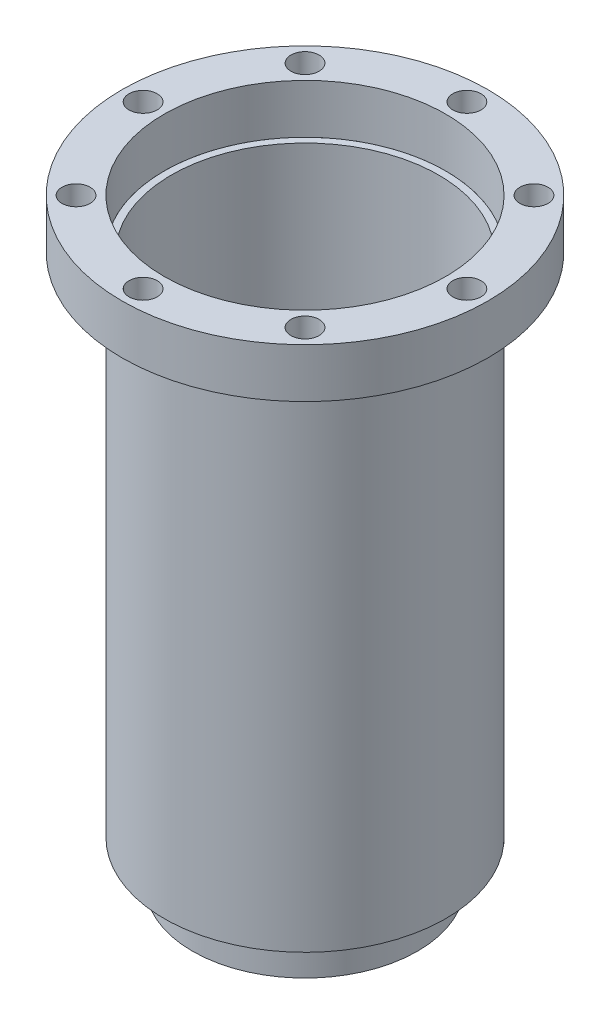
from build123d import *

# Parameters (mm, degrees)
SKETCH1_R               = 100
BOSS_EXTRUDE1_DEPTH     = 360
SHELL1_T                = -10
SKETCH2_R               = 70
CUT_EXTRUDE1_DEPTH      = 300
SKETCH3_R               = 80
SKETCH3_R_2             = 70
BOSS_EXTRUDE2_DEPTH     = 30
SKETCH4_R               = 130
SKETCH4_R_2             = 100
BOSS_EXTRUDE3_DEPTH     = 35
CUT_EXTRUDE3_DEPTH      = 432.161222746
CUT_EXTRUDE3_DEPTH_BACK = 309
SKETCH6_R               = 95
SKETCH6_R_2             = 90
SKETCH7_R               = 10
CUT_EXTRUDE6_DEPTH      = 464.060471213
CIRPATTERN1_COUNT       = 8


with BuildPart() as part:
    # Sketch1 → Boss-Extrude1 (new body)
    with BuildSketch(Plane(origin=(0, 0, 0), x_dir=(1, 0, 0), z_dir=(0, 1, 0))):
        with Locations(Location((0, 0, 0), (0, 0, 90))):
            Circle(SKETCH1_R)
    extrude(amount=BOSS_EXTRUDE1_DEPTH)

    # Shell1
    shell1_openings = [part.faces().sort_by_distance(p)[0] for p in [
        (0, 360, 0),
    ]]
    offset(amount=SHELL1_T, openings=shell1_openings, kind=Kind.INTERSECTION)

    # Sketch2 → Cut-Extrude1 (cut)
    with BuildSketch(Plane(origin=(0, 10, 0), x_dir=(1, 0, 0), z_dir=(0, 1, 0))):
        with Locations(Location((0, 0, 0), (0, 0, 270))):
            Circle(SKETCH2_R)
    extrude(amount=-CUT_EXTRUDE1_DEPTH, mode=Mode.SUBTRACT)

    # Sketch3 → Boss-Extrude2 (add)
    with BuildSketch(Plane.XZ):
        with Locations(Location((0, 0, 0), (0, 0, 90))):
            Circle(SKETCH3_R)
        with Locations(Location((0, 0, 0), (0, 0, 90))):
            Circle(SKETCH3_R_2, mode=Mode.SUBTRACT)
    extrude(amount=BOSS_EXTRUDE2_DEPTH)

    # Sketch6 → Cut-Extrude3 (cut, two sides: drawn at the far end of the back side and taken through both)
    with BuildSketch(Plane(origin=(0, 360, 0), x_dir=(1, 0, 0), z_dir=(0, 1, 0)).offset(-CUT_EXTRUDE3_DEPTH_BACK)):
        with Locations(Location((0, 0, 0), (0, 0, 270))):
            Circle(SKETCH6_R)
        with Locations(Location((0, 0, 0), (0, 0, 90))):
            Circle(SKETCH6_R_2, mode=Mode.SUBTRACT)
    extrude(amount=CUT_EXTRUDE3_DEPTH + CUT_EXTRUDE3_DEPTH_BACK, mode=Mode.SUBTRACT)


with BuildPart() as body_2:
    # Sketch4 → Boss-Extrude3 (new body)
    with BuildSketch(Plane(origin=(0, 360, 0), x_dir=(1, 0, 0), z_dir=(0, 1, 0))):
        with Locations(Location((0, 0, 0), (0, 0, 270))):
            Circle(SKETCH4_R)
        with Locations(Location((0, 0, 0), (0, 0, 270))):
            Circle(SKETCH4_R_2, mode=Mode.SUBTRACT)
    extrude(amount=BOSS_EXTRUDE3_DEPTH)

    # Sketch7 → Cut-Extrude6 (cut, symmetric)
    with BuildSketch(Plane(origin=(0, 395, 0), x_dir=(1, 0, 0), z_dir=(0, 1, 0))):
        with Locations(Location((-115, 0, 0), (0, 0, 270))):
            Circle(SKETCH7_R)
    cut_extrude6 = extrude(amount=CUT_EXTRUDE6_DEPTH, both=True, mode=Mode.SUBTRACT)

    # CirPattern1: Cut-Extrude6 ×8 about axis
    cirpattern1_axis = Axis((0, 0, 0), (0, 1, 0))
    for i in range(1, CIRPATTERN1_COUNT):
        add(cut_extrude6.rotate(cirpattern1_axis, i * 360 / CIRPATTERN1_COUNT), mode=Mode.SUBTRACT)


solid = Compound([part.part, body_2.part])
